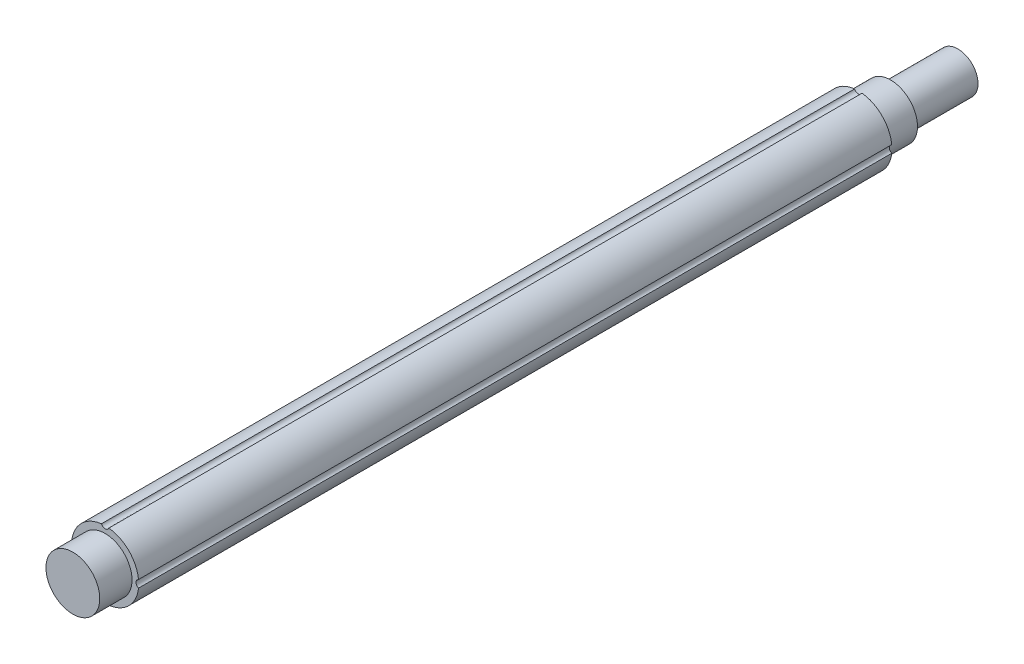
from build123d import *

# Parameters (mm, degrees)
SKETCH_1_R               = 12.5
EXTRUDE_1_DEPTH          = 280
SKETCH_2_R               = 10
EXTRUDE_2_DEPTH          = 12
EXTRUDE_START            = 12
SKETCH_3_R               = 10
EXTRUDE_3_DEPTH          = 12
SKETCH_4_R               = 7.5
EXTRUDE_4_DEPTH          = 25
SKETCH_5_R               = 1.5
CUT_EXTRUDE_1_DEPTH      = 280
PATTERN_CIRCULAR_1_COUNT = 4


with BuildPart() as part:
    # 草图1 → 凸台-拉伸1 (new body)
    with BuildSketch(Plane.XY):
        Circle(SKETCH_1_R)
    extrude(amount=EXTRUDE_1_DEPTH)

    # 草图2 → 凸台-拉伸2 (add)
    with BuildSketch(Plane.XY.offset(280)):
        Circle(SKETCH_2_R)
    extrude(amount=EXTRUDE_2_DEPTH)

    # 草图3 → 凸台-拉伸3 (add)
    with BuildSketch(Plane(origin=(0, 0, 0), x_dir=(-1, 0, 0), z_dir=(0, 0, -1)).offset(EXTRUDE_START)):
        with Locations(Location((0, 0, 0), (0, 0, 180))):
            Circle(SKETCH_3_R)
    extrude(amount=-EXTRUDE_3_DEPTH)

    # 草图4 → 凸台-拉伸4 (add)
    with BuildSketch(Plane(origin=(0, 0, -12), x_dir=(-1, 0, 0), z_dir=(0, 0, -1))):
        Circle(SKETCH_4_R)
    extrude(amount=EXTRUDE_4_DEPTH)

    # 草图5 → 切除-拉伸1 (cut)
    with BuildSketch(Plane(origin=(0, 0, 0), x_dir=(-1, 0, 0), z_dir=(0, 0, -1))):
        with Locations((0, 13)):
            Circle(SKETCH_5_R)
    cut_extrude_1 = extrude(amount=-CUT_EXTRUDE_1_DEPTH, mode=Mode.SUBTRACT)

    # 阵列(圆周)1: 切除-拉伸1 ×4 about axis
    pattern_circular_1_axis = Axis((0, 0, 0), (0, 0, 1))
    for i in range(1, PATTERN_CIRCULAR_1_COUNT):
        add(cut_extrude_1.rotate(pattern_circular_1_axis, i * 360 / PATTERN_CIRCULAR_1_COUNT), mode=Mode.SUBTRACT)


solid = part.part
